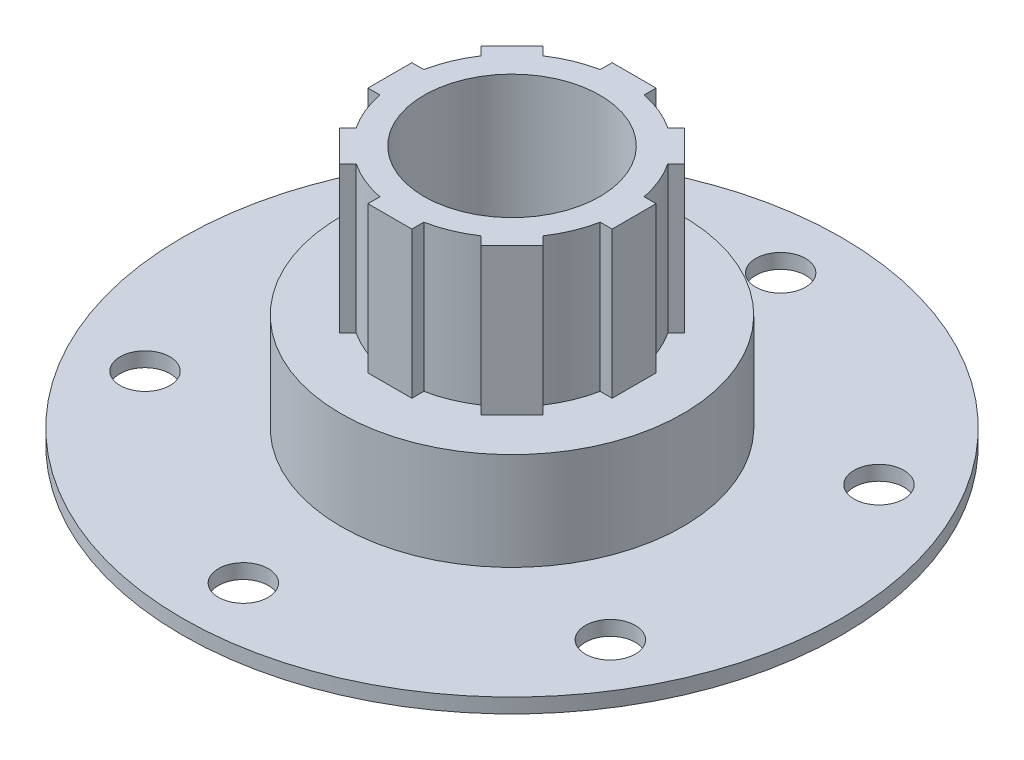
from build123d import *

# Parameters (mm, degrees)
SKETCH_1_R              = 67.5
SKETCH_1_R_2            = 18
EXTRUDE_1_DEPTH         = 53
SKETCH_2_OUTSIDE_W      = 176.628
SKETCH_2_OUTSIDE_H      = 176.628
SKETCH_2_OUTSIDE_R      = 35
CUT_EXTRUDE_1_DEPTH     = 50
SKETCH_3_OUTSIDE_W      = 176.628
SKETCH_3_OUTSIDE_H      = 176.628
SKETCH_3_OUTSIDE_R      = 23
CUT_EXTRUDE_2_DEPTH     = 30
EXTRUDE_2_DEPTH         = 30
HOLE_WIZARD_M12_1_D     = 10.2
HOLE_WIZARD_M12_1_DEPTH = 5
HOLE_WIZARD_M12_1_TIP   = 3.064389157


with BuildPart() as part:
    # 草图1 → 凸台-拉伸1 (new body)
    with BuildSketch(Plane(origin=(0, 0, 0), x_dir=(1, 0, 0), z_dir=(0, 1, 0))):
        with Locations(Location((0, 0, 0), (0, 0, 270))):
            Circle(SKETCH_1_R)
        with Locations(Location((0, 0, 0), (0, 0, 270))):
            Circle(SKETCH_1_R_2, mode=Mode.SUBTRACT)
    extrude(amount=EXTRUDE_1_DEPTH)

    # 草图2 outside → 切除-拉伸1 (cut)
    with BuildSketch(Plane(origin=(0, 53, 0), x_dir=(1, 0, 0), z_dir=(0, 1, 0))):
        Rectangle(SKETCH_2_OUTSIDE_W, SKETCH_2_OUTSIDE_H)
        with Locations(Location((0, 0, 0), (0, 0, 270))):
            Circle(SKETCH_2_OUTSIDE_R, mode=Mode.SUBTRACT)
    extrude(amount=-CUT_EXTRUDE_1_DEPTH, mode=Mode.SUBTRACT)

    # 草图3 outside → 切除-拉伸2 (cut)
    with BuildSketch(Plane(origin=(0, 53, 0), x_dir=(1, 0, 0), z_dir=(0, 1, 0))):
        Rectangle(SKETCH_3_OUTSIDE_W, SKETCH_3_OUTSIDE_H)
        with Locations(Location((0, 0, 0), (0, 0, 270))):
            Circle(SKETCH_3_OUTSIDE_R, mode=Mode.SUBTRACT)
    extrude(amount=-CUT_EXTRUDE_2_DEPTH, mode=Mode.SUBTRACT)

    # 草图4 → 凸台-拉伸2 (add)
    with BuildSketch(Plane(origin=(0, 53, 0), x_dir=(1, 0, 0), z_dir=(0, 1, 0))):
        Polygon((0, 25), (4.5, 25), (4.5, 18.659112383), (-4.5, 18.659112383), (-4.5, 25), align=None)
        Polygon((10.012004382, 16.375965412), (14.495689014, 20.859650045), (17.67766953, 17.67766953), (20.859650045, 14.495689014), (16.375965412, 10.012004382), align=None)
        Polygon((18.659112383, 4.5), (25, 4.5), (25, 0), (25, -4.5), (18.659112383, -4.5), align=None)
        Polygon((16.375965412, -10.012004382), (20.859650045, -14.495689014), (17.67766953, -17.67766953), (14.495689014, -20.859650045), (10.012004382, -16.375965412), align=None)
        Polygon((4.5, -18.659112383), (4.5, -25), (0, -25), (-4.5, -25), (-4.5, -18.659112383), align=None)
        Polygon((-10.012004382, -16.375965412), (-14.495689014, -20.859650045), (-17.67766953, -17.67766953), (-20.859650045, -14.495689014), (-16.375965412, -10.012004382), align=None)
        Polygon((-18.659112383, -4.5), (-25, -4.5), (-25, 0), (-25, 4.5), (-18.659112383, 4.5), align=None)
        Polygon((-16.375965412, 10.012004382), (-20.859650045, 14.495689014), (-17.67766953, 17.67766953), (-14.495689014, 20.859650045), (-10.012004382, 16.375965412), align=None)
    extrude(amount=-EXTRUDE_2_DEPTH)

    # M12 螺纹孔的螺纹孔钻头1
    with Locations(Plane(origin=(0, 3, 0), x_dir=(1, 0, 0), z_dir=(0, 1, 0))):
        with Locations((0, 55), (-47.631397208, 27.5), (-47.631397208, -27.5), (0, -55), (47.631397208, -27.5), (47.631397208, 27.5)):
            Hole(HOLE_WIZARD_M12_1_D / 2, depth=HOLE_WIZARD_M12_1_DEPTH)
            with Locations((0, 0, -(HOLE_WIZARD_M12_1_DEPTH + HOLE_WIZARD_M12_1_TIP / 2))):  # 118° drill point
                Cone(0, HOLE_WIZARD_M12_1_D / 2, HOLE_WIZARD_M12_1_TIP, mode=Mode.SUBTRACT)


solid = part.part
